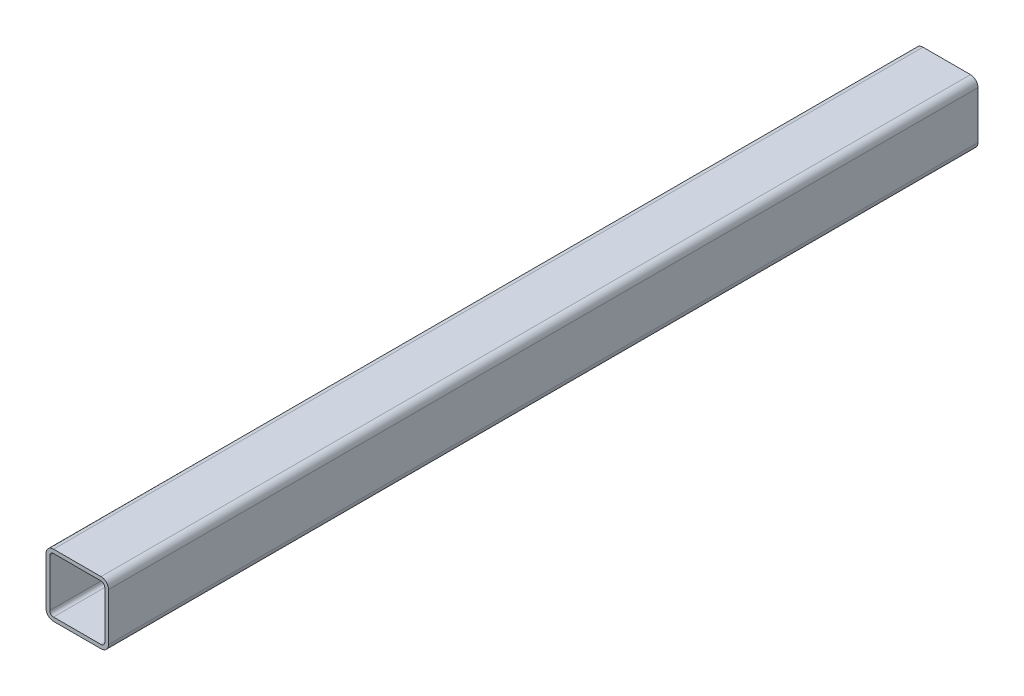
SolidWorks part; units mm, degrees
material "Q235B"
ref_plane "前视基准面" through (0, 0, 0) normal (0, 0, 1) x (1, 0, 0)
ref_plane "上视基准面" through (0, 0, 0) normal (0, 1, 0) x (1, 0, 0)
ref_plane "右视基准面" through (0, 0, 0) normal (1, 0, 0) x (0, 0, -1)
other "Configuration Table"
sketch "草图1" plane through (0, 0, 0) normal (1, 0, 0) x (0, 0, -1)
  line L0 (-347.5, 0) -> (347.5, 0)
other "Gb／6728-1986方形空心型钢 050 X 50 X 3(1)"
ref_plane "基准面1" through (0, 0, 347.5) normal (0, 0, -1) x (0, 1, 0)
sketch "Sketch1" plane through (0, 0, 347.5) normal (0, 0, -1) x (0, 1, 0)
  line L0 (-19, -22) -> (19, -22)
  line L1 (-22, -19) -> (-22, 19)
  line L2 (19, 22) -> (-19, 22)
  line L3 (22, 19) -> (22, -19)
  line L4 (-19, -25) -> (19, -25)
  line L5 (-25, -19) -> (-25, 19)
  line L6 (19, 25) -> (-19, 25)
  line L7 (25, 19) -> (25, -19)
  arc A0 (25, 19) -> (19, 25) centre (19, 19) ccw
  arc A1 (19, -25) -> (25, -19) centre (19, -19) ccw
  arc A2 (-25, -19) -> (-19, -25) centre (-19, -19) ccw
  arc A3 (-19, 25) -> (-25, 19) centre (-19, 19) ccw
  arc A4 (-19, 22) -> (-22, 19) centre (-19, 19) ccw
  arc A5 (22, 19) -> (19, 22) centre (19, 19) ccw
  arc A6 (19, -22) -> (22, -19) centre (19, -19) ccw
  arc A7 (-22, -19) -> (-19, -22) centre (-19, -19) ccw
  point P0 (-25, 0)
  point P1 (25, 0)
  point P2 (0, 25)
  point P3 (0, -25)
  point P4 (0, 0)
  point P5 (-25, -25)
  point P6 (25, -25)
  point P7 (25, 25)
  point P8 (-25, 25)
  point P33 (0, 0)
  dimension "D1" = 6
  dimension "Thickness" = 3
  dimension "V_leg" = 50
equation "\"D2@草图1\"=\"D1@草图1\"/2"
